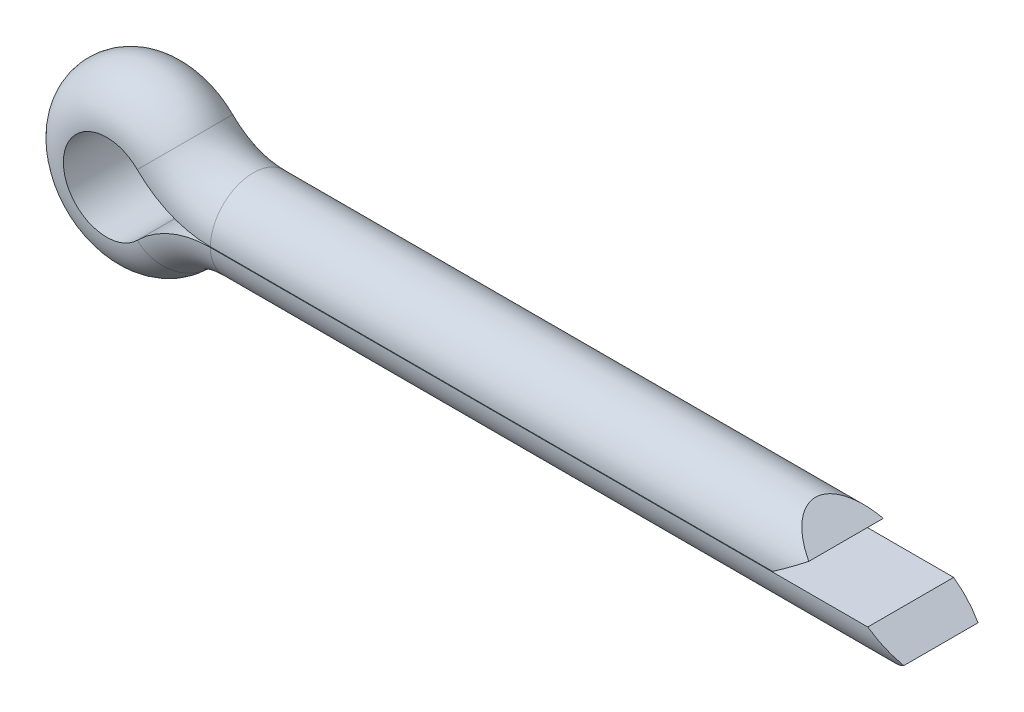
from build123d import *

# Parameters (mm, degrees)
CUT_EXTRUDE1_DEPTH      = 27.896141003
CUT_EXTRUDE1_DEPTH_BACK = 27.896141003


with BuildPart() as part:
    # Sweep2: sweep along a path in Dimension sketch
    with BuildLine(Plane.XY) as sweep2_path:
        Line((23.5, 1.45), (3.5, 1.45))
        ThreePointArc((3.5, 1.45), (2.715712277, 1.606029633), (2.050862219, 2.050357081))
        ThreePointArc((2.050862219, 2.050357081), (-2.9, 0), (2.050862219, -2.050357081))
        ThreePointArc((2.050862219, -2.050357081), (2.715712277, -1.606029633), (3.5, -1.45))
        Line((3.5, -1.45), (26.7, -1.45))
    # Sketch2 → Sweep2 (sweep)
    with BuildSketch(Plane(origin=(23.5, 1.45, 0), x_dir=(0, 0, 1), z_dir=(-1, 0, 0))):
        with BuildLine():
            Line((-1.449965517, -1.44), (1.449965517, -1.44))
            ThreePointArc((1.449965517, -1.44), (0, 0), (-1.449965517, -1.44))
        make_face()
    sweep(path=sweep2_path.line)

    # Sketch3 → Cut-Extrude1 (cut, two sides: drawn at the far end of the back side and taken through both)
    with BuildSketch(Plane.XY.offset(-CUT_EXTRUDE1_DEPTH_BACK)):
        Polygon((23.5, 0.72), (22.468093733, 1.45), (26.71, 1.45), (26.71, -1.45), (25.661091657, -1.45), (26.7, -0.73), (25.668093733, 0), (22.461091657, 0), align=None)
    extrude(amount=CUT_EXTRUDE1_DEPTH + CUT_EXTRUDE1_DEPTH_BACK, mode=Mode.SUBTRACT)


solid = part.part
